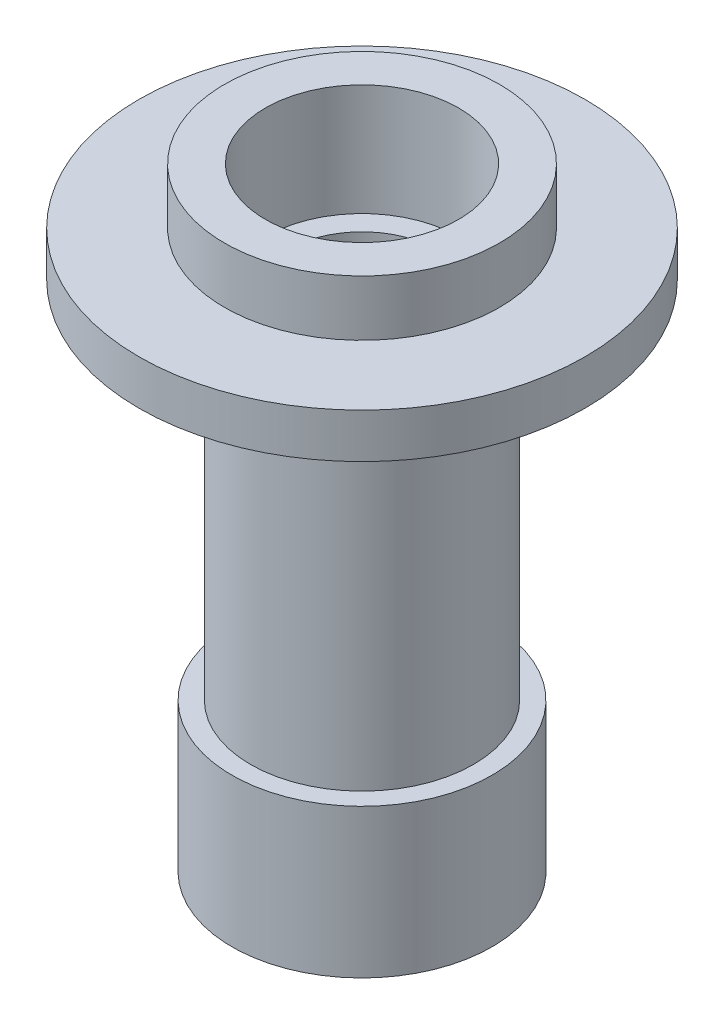
SolidWorks part; units mm, degrees
ref_plane "Front Plane" through (0, 0, 0) normal (0, 0, 1) x (1, 0, 0)
ref_plane "Top Plane" through (0, 0, 0) normal (0, 1, 0) x (1, 0, 0)
ref_plane "Right Plane" through (0, 0, 0) normal (1, 0, 0) x (0, 0, -1)
ref_plane "Plane1" through (0, 0, -440.693) normal (0, 0, 1) x (1, 0, 0)
sketch "Sketch1" plane through (0, 0, -440.693) normal (0, 0, 1) x (1, 0, 0)
  line L0 (551.2306, 721.8956) -> (551.2306, 804.8956)
  line L1 (551.2306, 804.8956) -> (556.2306, 804.8956)
  line L2 (556.2306, 804.8956) -> (556.2306, 819.8956)
  line L3 (556.2306, 819.8956) -> (581.2306, 819.8956)
  line L4 (581.2306, 819.8956) -> (581.2306, 831.8956)
  line L5 (581.2306, 831.8956) -> (558.2306, 831.8956)
  line L6 (558.2306, 831.8956) -> (558.2306, 846.8956)
  line L7 (558.2306, 846.8956) -> (547.2306, 846.8956)
  line L8 (547.2306, 846.8956) -> (547.2306, 816.8956)
  line L9 (547.2306, 816.8956) -> (541.2306, 816.8956)
  line L10 (541.2306, 816.8956) -> (541.2306, 701.8956)
  line L11 (541.2306, 701.8956) -> (547.2306, 701.8956)
  line L12 (547.2306, 701.8956) -> (547.2306, 681.8956)
  line L13 (547.2306, 681.8956) -> (556.2306, 681.8956)
  line L14 (556.2306, 681.8956) -> (556.2306, 721.8956)
  line L15 (556.2306, 721.8956) -> (551.2306, 721.8956)
  line L16 (521.2306, 846.8956) -> (521.2306, 681.8956) construction
  dimension "D1" = 20
  dimension "D2" = 26
  dimension "D3" = 30
  dimension "D4" = 35
  dimension "D5" = 37
  dimension "D6" = 60
  dimension "D7" = 20
  dimension "D8" = 40
  dimension "D9" = 123
  dimension "D10" = 135
  dimension "D11" = 138
  dimension "D12" = 150
  dimension "D13" = 165
revolve "Revolve1" add sketch "Sketch1" angle 360 about L16
